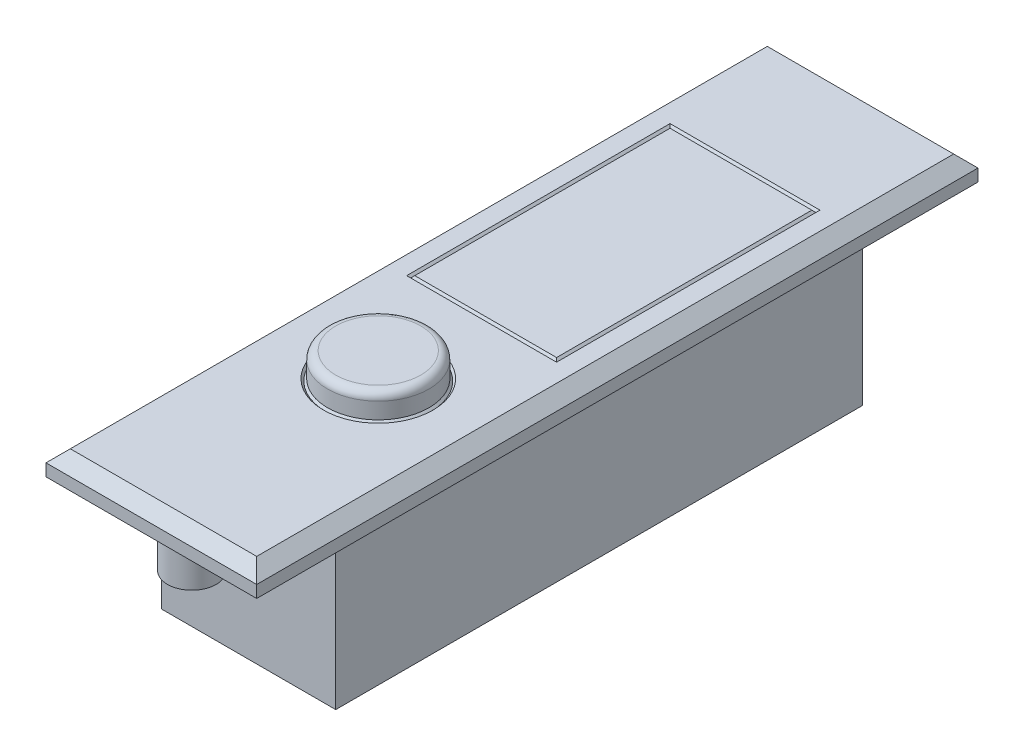
SolidWorks part; units mm, degrees
material "合金钢"
ref_plane "Front Plane" through (0, 0, 0) normal (0, 0, 1) x (1, 0, 0)
ref_plane "Top Plane" through (0, 0, 0) normal (0, 1, 0) x (1, 0, 0)
ref_plane "Right Plane" through (0, 0, 0) normal (1, 0, 0) x (0, 0, -1)
sketch "Sketch1" plane through (0, 0, 0) normal (0, 1, 0) x (1, 0, 0)
  line L1 (-13, 44.5) -> (13, 44.5)
  line L2 (-13, 44.5) -> (-13, -44.5)
  line L3 (-13, -44.5) -> (13, -44.5)
  line L4 (13, 44.5) -> (13, -44.5)
  line L5 (-13, 44.5) -> (13, -44.5) construction
  line L6 (-13, -44.5) -> (13, 44.5) construction
  point P0 (0, 0)
  dimension "D1" = 26
  dimension "D2" = 89
extrude "Boss-Extrude1" add sketch "Sketch1" along normal blind 3
sketch "Sketch2" plane through (0, 3, 0) normal (0, 1, 0) x (1, 0, 0)
  line L0 (13, 44.5) -> (-13, 44.5) construction
  line L1 (-9, 28.5) -> (9, 28.5)
  line L2 (-9, 28.5) -> (-9, -3.5)
  line L3 (-9, -3.5) -> (9, -3.5)
  line L4 (9, 28.5) -> (9, -3.5)
  line L5 (-9, 28.5) -> (9, -3.5) construction
  line L6 (-9, -3.5) -> (9, 28.5) construction
  line L7 (0, 47.7415) -> (0, -47.2416) construction
  line L8 (-13, -44.5) -> (13, -44.5) construction
  circle A0 centre (0, -16.5) radius 6.5
  point P0 (0, 12.5)
  dimension "D4" = 13
  dimension "D1" = 16
  dimension "D2" = 18
  dimension "D3" = 32
  dimension "D5" = 28
extrude "Cut-Extrude-Thin1" cut sketch "Sketch2" against normal blind 1 draft 44 thin
sketch "Sketch3" plane through (0, 3, 0) normal (0, 1, 0) x (1, 0, 0)
  circle A0 centre (0, -16.5) radius 6.25
extrude "Boss-Extrude2" add sketch "Sketch3" along normal blind 3
fillet "Fillet1" radius 1 1 edges at (0, 6, 22.75)
chamfer "Chamfer1" distance 1.5 angle 45 4 edges at (0, 3, -44.5) (13, 3, 0) (0, 3, 44.5) (-13, 3, 0)
sketch "Sketch4" plane through (0, 0, 0) normal (0, -1, 0) x (1, 0, 0)
  line L0 (0, -46.7167) -> (0, 54.8087) construction
  circle A0 centre (0, -39.5) radius 3
  circle A1 centre (0, 39.5) radius 3
  dimension "D3" = 6
  dimension "D4" = 6
  dimension "D1" = 79
  dimension "D2" = 39.5
extrude "Extrude-Thin2" add sketch "Sketch4" along normal blind 6 thin thin type one direction reverse wall 1
sketch "Sketch5" plane through (0, 0, 0) normal (0, -1, 0) x (1, 0, 0)
  line L1 (10.75, -32.5) -> (-10.75, -32.5)
  line L2 (10.75, -32.5) -> (10.75, 32.5)
  line L3 (10.75, 32.5) -> (-10.75, 32.5)
  line L4 (-10.75, -32.5) -> (-10.75, 32.5)
  line L5 (10.75, -32.5) -> (-10.75, 32.5) construction
  line L6 (10.75, 32.5) -> (-10.75, -32.5) construction
  point P0 (0, 0)
  dimension "D1" = 21.5
  dimension "D2" = 65
extrude "Boss-Extrude3" add sketch "Sketch5" along normal blind 19
